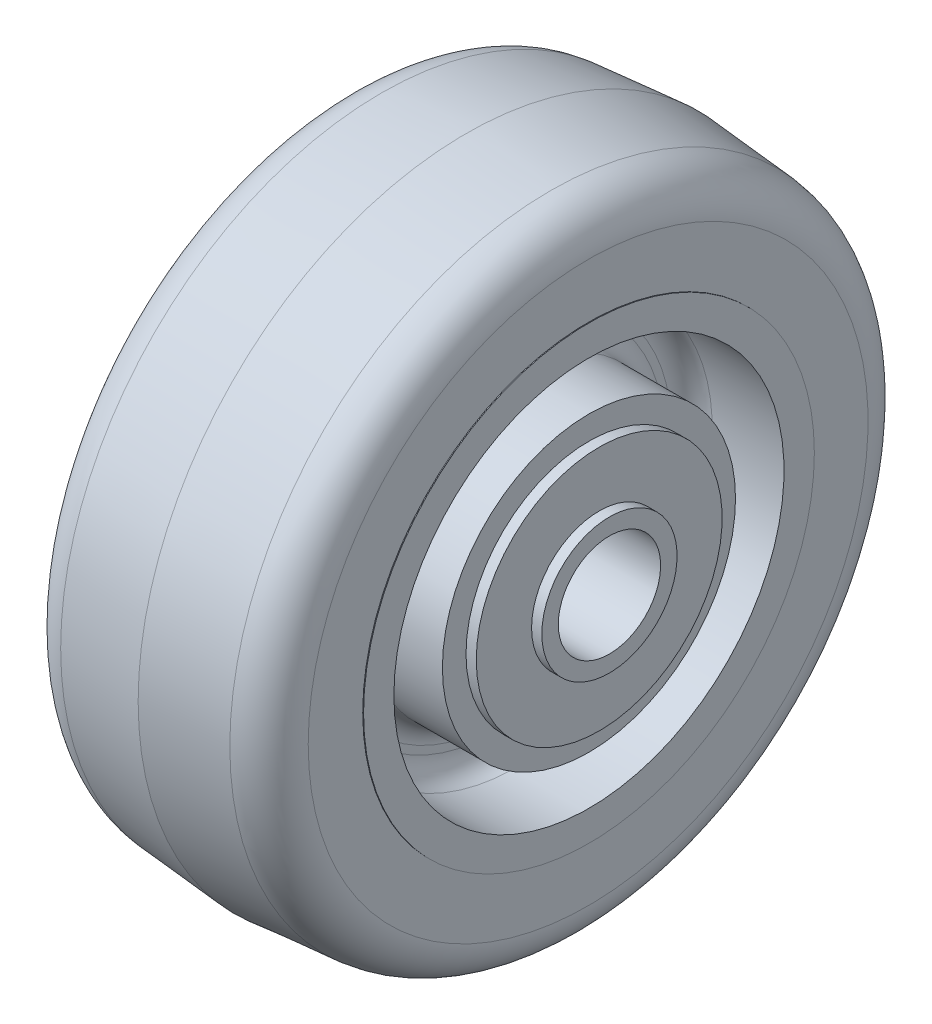
SolidWorks part; units mm, degrees
material "6061-T6 (SS)"
ref_plane "Front" through (0, 0, 0) normal (0, 0, 1) x (1, 0, 0)
ref_plane "Top" through (0, 0, 0) normal (0, 1, 0) x (1, 0, 0)
ref_plane "Right" through (0, 0, 0) normal (1, 0, 0) x (0, 0, -1)
sketch "Sketch3" plane through (0, 0, 0) normal (0, 0, 1) x (1, 0, 0)
  line L0 (-22.225, 7.9248) -> (-9.525, 7.9248)
  line L1 (0, 0) -> (0, 7.9248) construction
  line L2 (-32.0066, 0) -> (35.3235, 0) construction
  line L3 (-19.05, 34.925) -> (-19.05, 30.226)
  line L4 (-19.05, 30.226) -> (-7.9375, 30.226)
  line L5 (-4.7625, 27.051) -> (-4.7625, 25.8826)
  line L6 (-7.9375, 22.7076) -> (-19.05, 22.7076)
  line L7 (-19.05, 22.7076) -> (-19.05, 19.05)
  line L8 (-9.525, 12.7) -> (9.525, 12.7)
  line L9 (-9.525, 12.7) -> (-9.525, 7.9248)
  line L10 (-13.104, 49.7003) -> (0, 50.8)
  line L11 (19.05, 34.925) -> (18.923, 34.925)
  line L12 (-19.05, 34.925) -> (-18.923, 34.925)
  line L13 (-18.923, 34.925) -> (-18.923, 43.3725)
  line L14 (-19.05, 19.05) -> (-20.6375, 19.05)
  line L15 (-20.6375, 19.05) -> (-20.6375, 10.4775)
  line L16 (-20.6375, 10.4775) -> (-22.225, 10.4775)
  line L17 (-22.225, 10.4775) -> (-22.225, 7.9248)
  line L18 (9.525, 12.7) -> (9.525, 7.9248)
  line L19 (9.525, 7.9248) -> (22.225, 7.9248)
  line L20 (22.225, 10.4775) -> (22.225, 7.9248)
  line L21 (20.6375, 10.4775) -> (22.225, 10.4775)
  line L22 (20.6375, 19.05) -> (20.6375, 10.4775)
  line L23 (19.05, 19.05) -> (20.6375, 19.05)
  line L24 (19.05, 22.7076) -> (19.05, 19.05)
  line L25 (7.9375, 22.7076) -> (19.05, 22.7076)
  line L26 (4.7625, 27.051) -> (4.7625, 25.8826)
  line L27 (19.05, 34.925) -> (19.05, 30.226)
  line L28 (19.05, 30.226) -> (7.9375, 30.226)
  line L29 (18.923, 34.925) -> (18.923, 43.3725)
  line L30 (13.104, 49.7003) -> (0, 50.8)
  arc A0 (-7.9375, 22.7076) -> (-4.7625, 25.8826) centre (-7.9375, 25.8826) ccw
  arc A1 (-4.7625, 27.051) -> (-7.9375, 30.226) centre (-7.9375, 27.051) ccw
  arc A2 (-13.104, 49.7003) -> (-18.923, 43.3725) centre (-12.573, 43.3725) ccw
  arc A3 (7.9375, 22.7076) -> (4.7625, 25.8826) centre (7.9375, 25.8826) cw
  arc A4 (4.7625, 27.051) -> (7.9375, 30.226) centre (7.9375, 27.051) cw
  arc A5 (13.104, 49.7003) -> (18.923, 43.3725) centre (12.573, 43.3725) cw
  point P30 (-18.923, 49.2119)
  dimension "D17" = 3.175
  dimension "D18" = 6.35
  dimension "D2" = 7.9248
  dimension "D3" = 30.226
  dimension "D4" = 22.7076
  dimension "D5" = 14.2875
  dimension "D6" = 69.85
  dimension "D7" = 101.6
  dimension "D8" = 14.2875
  dimension "D9" = 0.127
  dimension "D10" = 38.1
  dimension "D11" = 1.5875
  dimension "D12" = 20.955
  dimension "D13" = 19.05
  dimension "D14" = 9.525
  dimension "D16" = 25.4
revolve "Revolve1" add sketch "Sketch3" angle 360 about L2
